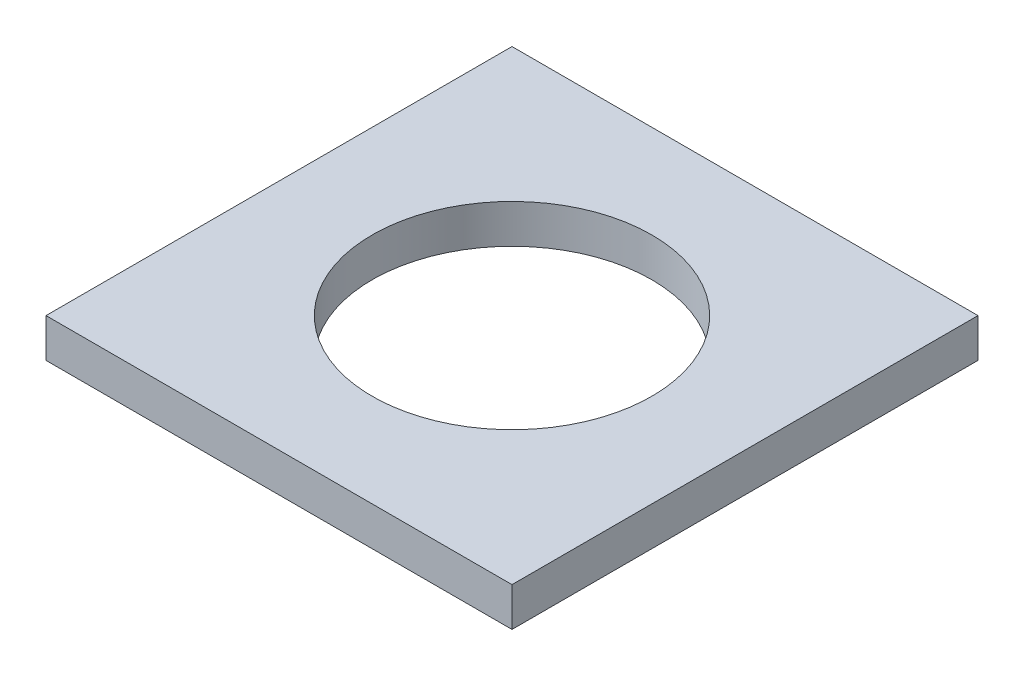
from build123d import *

# Parameters (mm, degrees)
SKETCH1_W           = 120
SKETCH1_H           = 120
SKETCH1_R           = 36
BOSS_EXTRUDE1_DEPTH = 10


with BuildPart() as part:
    # Sketch1 → Boss-Extrude1 (new body)
    with BuildSketch(Plane(origin=(0, 819.895595987, 0), x_dir=(1, 0, 0), z_dir=(0, 1, 0))):
        with Locations((521.230642584, 440.692981355)):
            Rectangle(SKETCH1_W, SKETCH1_H)
        with Locations(Location((521.230642584, 440.692981355, 0), (0, 0, 90))):
            Circle(SKETCH1_R, mode=Mode.SUBTRACT)
    extrude(amount=-BOSS_EXTRUDE1_DEPTH)


solid = part.part
